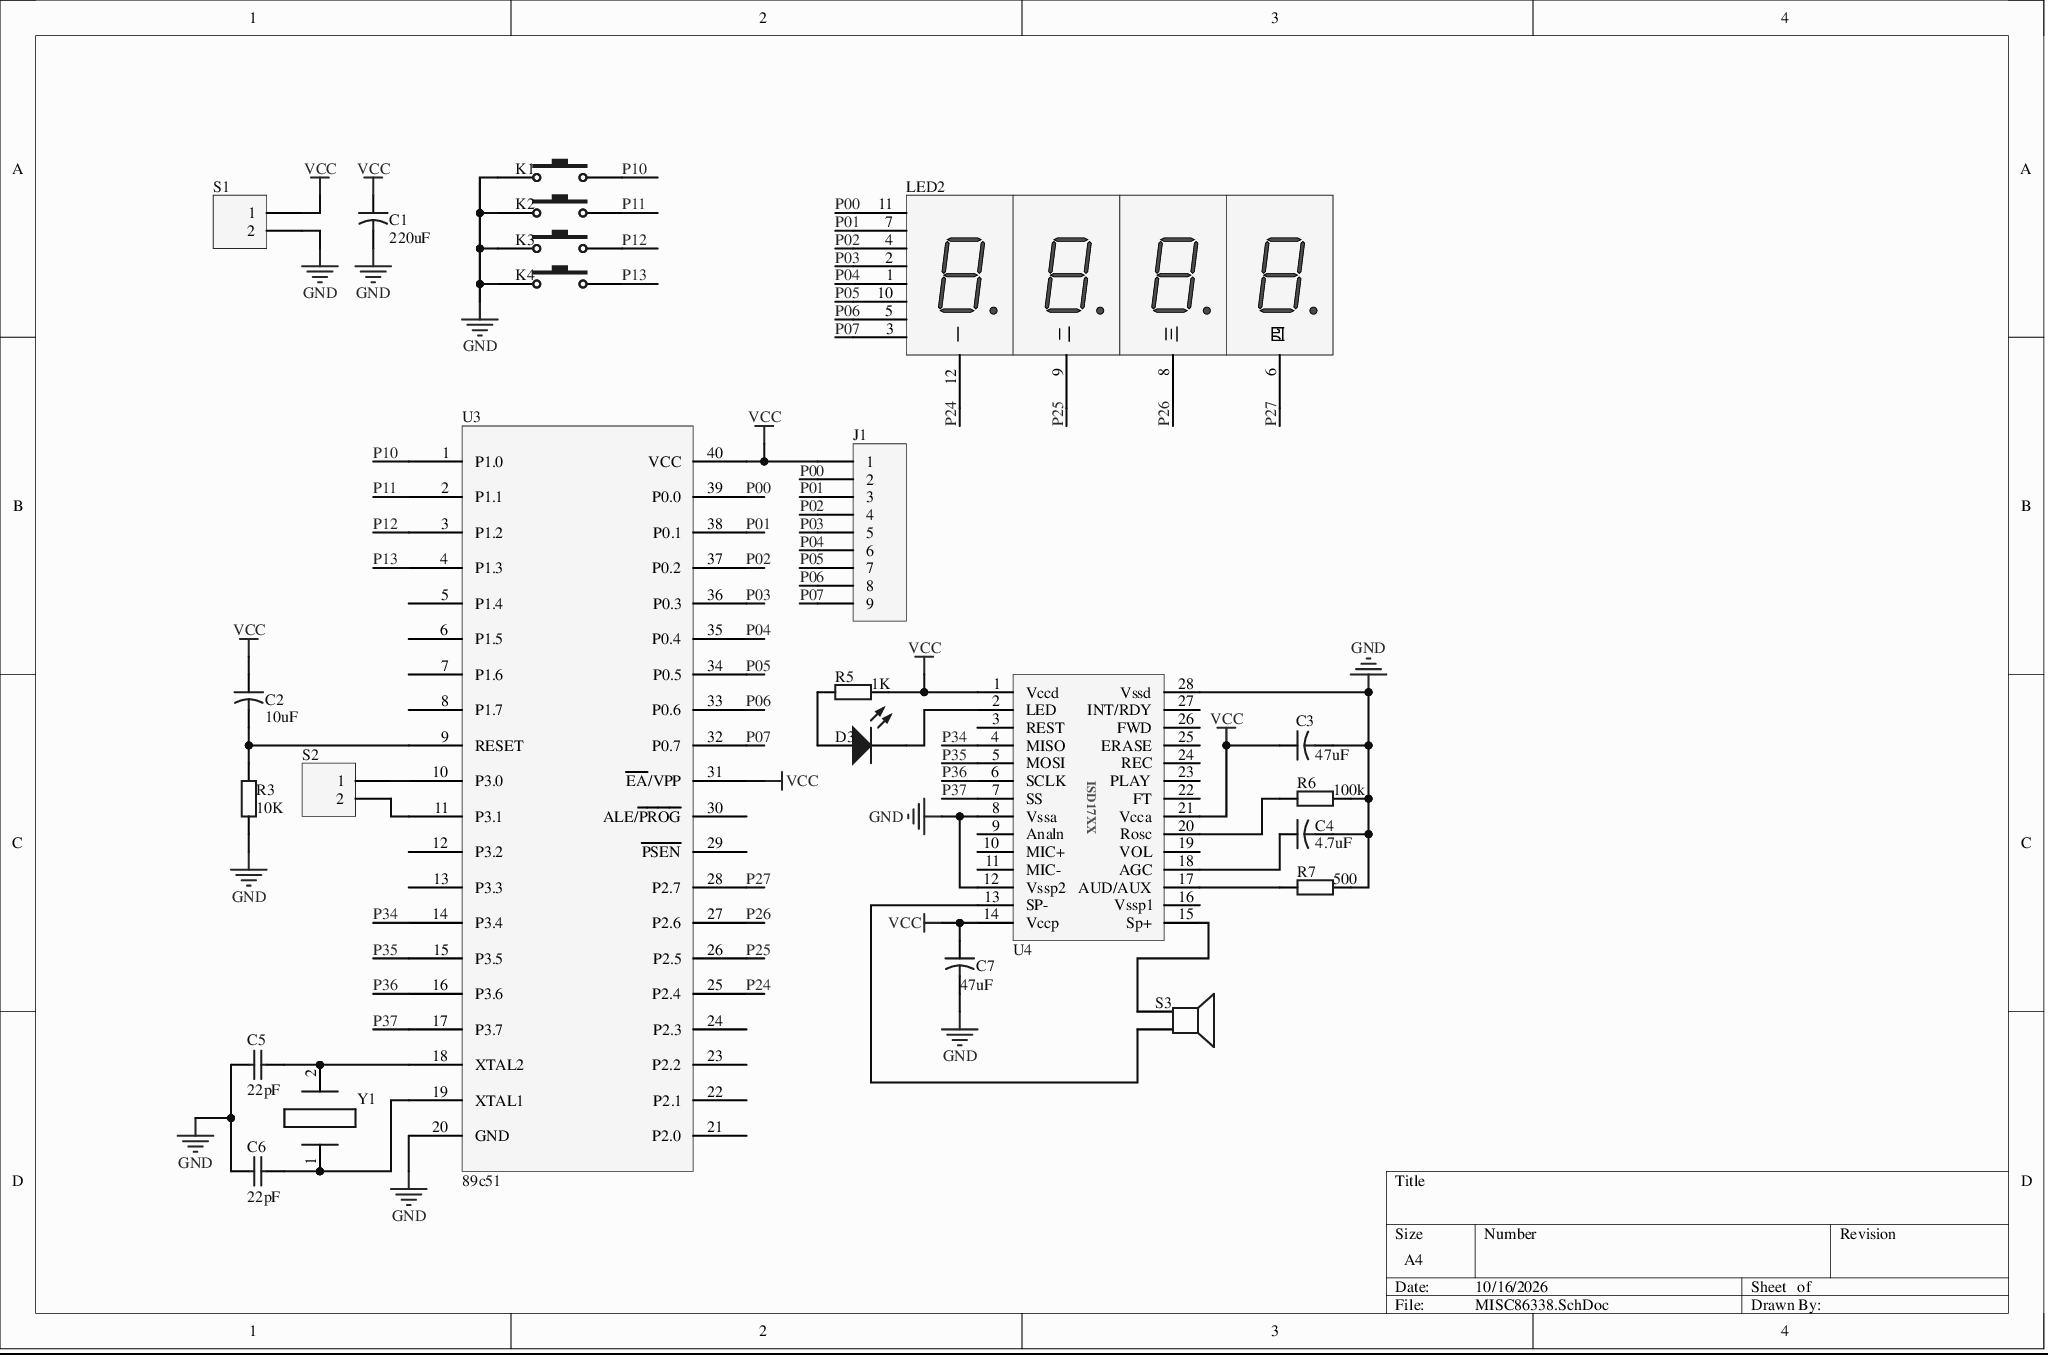
[diagram p0: MISC86338.SchDoc]
# Altium project MISC86338.PrjPcb
1 sheet, 24 parts. Net scope: global (net labels, ports and power ports of the same name join across sheets).
Board file: MISC86338.PcbDoc

## Sheet MISC86338.SchDoc
size A4

### Parts
C1  value 220uF  [CAPR5-4X5]  (hidden comment: Cap2)
C2  value 10uF  [CAPR5-4X5]  (hidden comment: Cap2)
C3  value 47uF  [CAPR5-4X5]  (hidden comment: Cap2)
C4  value 4.7uF  [CAPR5-4X5]  (hidden comment: Cap2)
C5  value 22pF  [RAD-0.3]  (hidden comment: Cap)
C6  value 22pF  [RAD-0.3]  (hidden comment: Cap)
C7  value 47uF  [CAPR5-4X5]  (hidden comment: Cap2)
D3  LED1  [LED-1]  (value not drawn)
J1  Header 9  [HDR1X9]  (value not drawn)
K1  SW-PB  [SPST-2]  (value not drawn)
K2  SW-PB  [SPST-2]  (value not drawn)
K3  SW-PB  [SPST-2]  (value not drawn)
K4  SW-PB  [SPST-2]  (value not drawn)
LED2  Dpy Red-CA  [四位数码管]  (value not drawn)
R3  value 10K  [AXIAL-0.4]  (hidden comment: Res2)
R5  value 1K  [AXIAL-0.4]  (hidden comment: Res2)
R6  value 100k  [AXIAL-0.4]  (hidden comment: Res2)
R7  value 500  [AXIAL-0.4]  (hidden comment: Res2)
S1  Header 2  [HDR1X2]  (value not drawn)
S2  Header 2  [HDR1X2]  (value not drawn)
S3  Speaker  [PIN2]  (value not drawn)
U3  89c51  [89c51]
U4  Component_1  [ISD1730]  (value not drawn)
Y1  Component_1  [XTAL]  (value not drawn)

### Nets
GND: C1.2 C3.2 C4.2 C5.1 C6.1 C7.2 K1.1 K2.1 K3.1 K4.1 R3.1 R6.1 R7.1 S1.2 U3.20(GND) U4.8(Vssa) U4.12(Vssp2) U4.28(Vssd)
VCC: C1.1 C2.1 C3.1 C7.1 J1.1 R5.1 S1.1 U3.31(~{EA}/VPP) U3.40(VCC) U4.1(Vccd) U4.14(Vccp) U4.21(Vcca)
P00: J1.2 LED2.11 U3.39(P0.0)
P01: J1.3 LED2.7 U3.38(P0.1)
P02: J1.4 LED2.4 U3.37(P0.2)
P03: J1.5 LED2.2 U3.36(P0.3)
P04: J1.6 LED2.1 U3.35(P0.4)
P05: J1.7 LED2.10 U3.34(P0.5)
P06: J1.8 LED2.5 U3.33(P0.6)
P07: J1.9 LED2.3 U3.32(P0.7)
P10: K1.2 U3.1(P1.0)
P11: K2.2 U3.2(P1.1)
P12: K3.2 U3.3(P1.2)
P13: K4.2 U3.4(P1.3)
P24: LED2.12(一) U3.25(P2.4)
P25: LED2.9(二) U3.26(P2.5)
P26: LED2.8(三) U3.27(P2.6)
P27: LED2.6(四) U3.28(P2.7)
P34: U3.14(P3.4) U4.4(MISO)
P35: U3.15(P3.5) U4.5(MOSI)
P36: U3.16(P3.6) U4.6(SCLK)
P37: U3.17(P3.7) U4.7(SS)
NetC2_2: C2.2 R3.2 U3.9(RESET)
NetC4_1: C4.1 U4.18(AGC)
NetC5_2: C5.2 U3.18(XTAL2) Y1.2
NetC6_2: C6.2 U3.19(XTAL1) Y1.1
NetD3_1: D3.1(A) R5.2
NetD3_2: D3.2(K) U4.2(LED)
NetR6_2: R6.2 U4.20(Rosc)
NetR7_2: R7.2 U4.17(AUD/AUX)
NetS2_1: S2.1 U3.10(P3.0)
NetS2_2: S2.2 U3.11(P3.1)
NetS3_1: S3.1 U4.15(Sp+)
NetS3_2: S3.2 U4.13(SP-)

Not connected (* = marked no-connect by the designer): U3 5(P1.4) 6(P1.5) 7(P1.6) 8(P1.7) 12(P3.2) 13(P3.3) 21(P2.0) 22(P2.1) 23(P2.2) 24(P2.3) 29(~{PSEN}) 30(ALE/~{PROG}); U4 3(REST) 9(Analn) 10(MIC+) 11(MIC-) 16(Vssp1) 19(VOL) 22(FT) 23(PLAY) 24(REC) 25(ERASE) 26(FWD) 27(INT/RDY)

### Library data of the parts
C1-C4 C7 = Cap2: Capacitor; Published: 23-Sep-2002; PackageReference: CAPR5-4X5; PackageDescription: Capacitor; 2 Leads; Publisher: Altium Limited
C5 C6 = Cap: Capacitor; Published: 8-Jun-2000; LatestRevisionDate: 17-Jul-2002; LatestRevisionNote: Re-released for DXP Platform.; PackageReference: RAD-0.3; PackageDescription: Radial Cap, Thru-Hole; 2 Leads; 0.3 in Pin Spacing; Publisher: Altium Limited
D3 = LED1: Typical RED GaAs LED; Published: 8-Jun-2000; LatestRevisionDate: 08-Jul-2005; LatestRevisionNote: Mech Layer 1 removed.; PackageReference: LED-1; PackageDescription: LED; 2 Leads; Publisher: Altium Limited
J1 = Header 9: Header, 9-Pin; LatestRevisionDate: 17-Jul-2002; LatestRevisionNote: Re-released for DXP Platform.; Publisher: Altium Limited
K1-K4 = SW-PB: Switch; Published: 24-Mar-1999; LatestRevisionDate: 17-Jul-2002; LatestRevisionNote: Re-released for DXP Platform.; PackageReference: SPST-2; PackageDescription: Switch; 2 Leads; Publisher: Altium Limited
LED2 = Dpy Red-CA: 7.62 mm Black Surface HER 7-Segment Display: CA, RH DP; MinimumIntensity: 360 ucd; Note: IF = 5 mA; Colour: High Efficiency Red (HER); Note: Pins 1 and 6 are redundant Anodes.; Published: 8-Jun-2000; LatestRevisionDate: 17-Dec-2003; LatestRevisionNote: Schematic revised, PCB Footprint replaced.; DatasheetVersion: 19-Feb-2002; PackageVersion: 11-Feb-2002; PackageReference: A; PackageDescription: LED, 7-Segment Display, 7.62 mm, RHD; 10 Leads; Row Space 5.08 mm; Pitch 2.54 mm; ComponentLink1Description: Manufacturer Link; Publisher: Altium Limited
R3 R5-R7 = Res2: Resistor; Published: 8-Jun-2000; LatestRevisionDate: 17-Jul-2002; LatestRevisionNote: Re-released for DXP Platform.; PackageReference: AXIAL-0.4; PackageDescription: Axial Device, Thru-Hole; 2 Leads; 0.4 in Pin Spacing; Publisher: Altium Limited
S1 S2 = Header 2: Header, 2-Pin; LatestRevisionDate: 17-Jul-2002; LatestRevisionNote: Re-released for DXP Platform.; Publisher: Altium Limited
S3 = Speaker: Loudspeaker; Published: 24-Mar-1999; LatestRevisionDate: 17-Jul-2002; LatestRevisionNote: Re-released for DXP Platform.; PackageReference: PIN2; Publisher: Altium Limited
U3 = Component_1